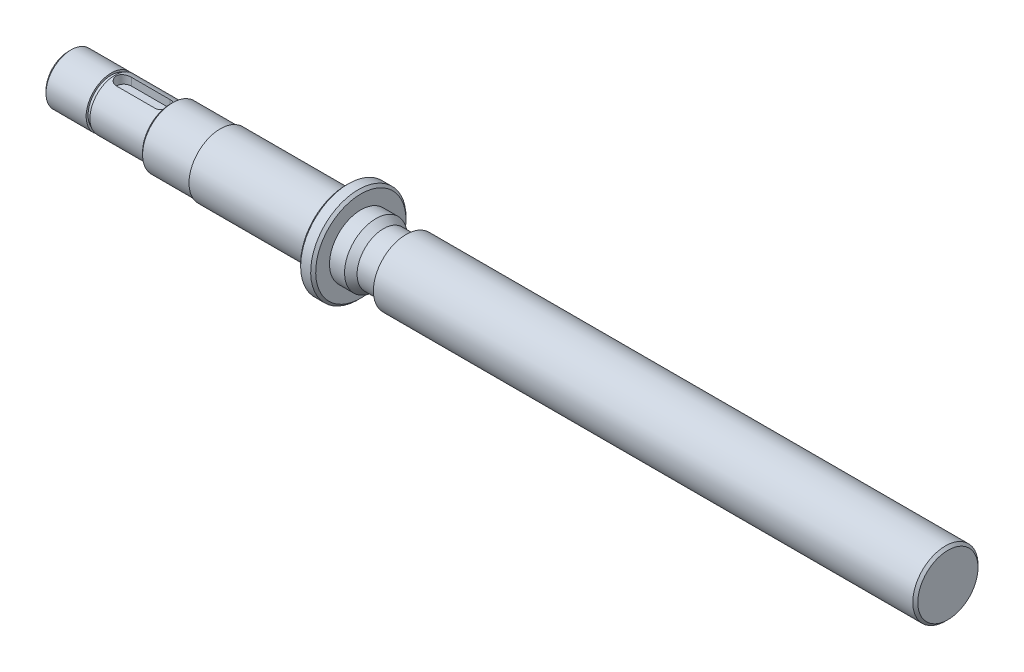
SolidWorks part; units mm, degrees
ref_plane "前视基准面" through (0, 0, 0) normal (0, 0, 1) x (1, 0, 0)
ref_plane "上视基准面" through (0, 0, 0) normal (0, 1, 0) x (1, 0, 0)
ref_plane "右视基准面" through (0, 0, 0) normal (1, 0, 0) x (0, 0, -1)
other "Configuration Table"
sketch "草图1" plane through (0, 0, 0) normal (0, 0, 1) x (1, 0, 0)
  line L0 (0, 0) -> (0, 10)
  line L1 (0, 10) -> (17, 10)
  line L2 (17, 10) -> (17, 9.25)
  line L3 (17, 9.25) -> (18.5, 9.25)
  line L4 (18.5, 9.25) -> (18.5, 10)
  line L5 (18.5, 10) -> (40.5, 10)
  line L6 (40.5, 10) -> (40.5, 12)
  line L7 (40.5, 12) -> (60.5, 12)
  line L8 (60.5, 12) -> (60.5, 12.5)
  line L9 (60.5, 12.5) -> (110.5, 12.5)
  line L10 (110.5, 12.5) -> (110.5, 19)
  line L11 (110.5, 19) -> (116.5, 19)
  line L12 (116.5, 19) -> (116.5, 12.5)
  line L13 (116.5, 12.5) -> (122.5, 12.5)
  line L14 (122.5, 12.5) -> (125.5, 10.5)
  line L15 (125.5, 10.5) -> (134.5, 10.5)
  line L16 (134.5, 10.5) -> (134.5, 13)
  line L17 (134.5, 13) -> (350.5, 13)
  line L18 (350.5, 13) -> (350.5, 0)
  line L19 (350.5, 0) -> (0, 0) construction
  line L20 (0, 0) -> (350.5, 0)
  dimension "D1" = 18.5
  dimension "D2" = 20
  dimension "D3" = 38
  dimension "D4" = 20
  dimension "D5" = 25
  dimension "D6" = 24
  dimension "D7" = 21
  dimension "D8" = 26
  dimension "D9" = 17
  dimension "D10" = 1.5
  dimension "D11" = 22
  dimension "D12" = 3
  dimension "D13" = 216
  dimension "D14" = 234
  dimension "D15" = 6
  dimension "D16" = 20
  dimension "D17" = 6
  dimension "D18" = 50
revolve "旋转1" add sketch "草图1" angle 360 about L19
cosmetic thread "装饰螺纹线1" parameters "D2"=20.752
cosmetic thread "装饰螺纹线2" parameters "D2"=17.294
cosmetic thread "装饰螺纹线3" parameters "D2"=20.752
ref_plane "基准面1" through (0, -10, 0) normal (0, 1, 0) x (1, 0, 0)
ref_plane "基准面2" through (0, 6.5, 0) normal (0, 1, 0) x (1, 0, 0)
sketch "草图2" plane through (0, 6.5, 0) normal (0, 1, 0) x (1, 0, 0)
  line L0 (22, 0) -> (37.5, 0) construction
  line L1 (22, 3) -> (37.5, 3)
  line L2 (22, -3) -> (37.5, -3)
  line L3 (40.5, 10) -> (40.5, -10) construction
  arc A0 (22, 3) -> (22, -3) centre (22, 0) ccw
  arc A1 (37.5, -3) -> (37.5, 3) centre (37.5, 0) ccw
  point P3 (29.75, 0)
  dimension "D1" = 3
  dimension "D2" = 15.5
extrude "切除-拉伸3" cut sketch "草图2" along normal through all
chamfer "倒角1" distance 1 angle 45 5 edges at (350.5, 13, 0) (116.5, 19, 0) (110.5, 19, 0) (40.5, 12, 0) (0, 10, 0)
